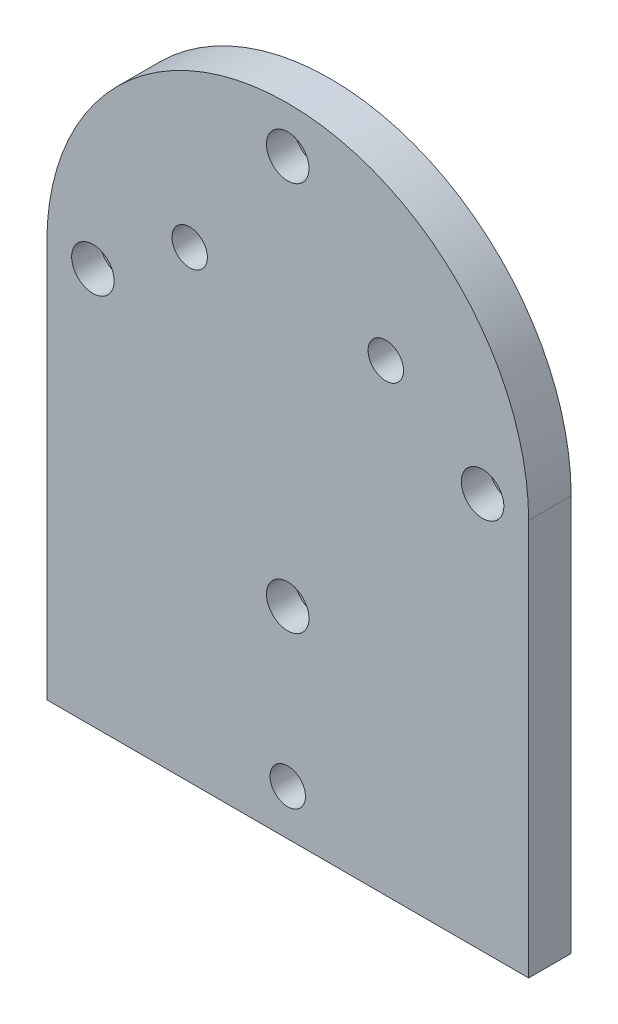
from build123d import *

# Parameters (mm, degrees)
BOSS_EXTRUDE1_DEPTH = 6
SKETCH3_R           = 3
CUT_EXTRUDE1_DEPTH  = 4
SKETCH9_R           = 2.5
CUT_EXTRUDE2_DEPTH  = 6


with BuildPart() as part:
    # Sketch2 → Boss-Extrude1 (new body)
    with BuildSketch(Plane.XY):
        with BuildLine():
            Line((2.181579686, 9.743947498), (2.181579686, -46.182702418))
            Line((2.181579686, -46.182702418), (-65.818420314, -46.182702418))
            Line((-65.818420314, -46.182702418), (-65.818420314, 9.743947498))
            ThreePointArc((-65.818420314, 9.743947498), (-31.818420314, 43.743947498), (2.181579686, 9.743947498))
        make_face()
    extrude(amount=BOSS_EXTRUDE1_DEPTH)

    # Sketch3 → Cut-Extrude1 (cut)
    with BuildSketch(Plane.XY.offset(6)):
        with Locations((-4.318420314, 9.743947498)):
            Circle(SKETCH3_R)
        with Locations((-31.818420314, -17.756052502)):
            Circle(SKETCH3_R)
        with Locations((-59.318420314, 9.743947498)):
            Circle(SKETCH3_R)
        with Locations((-31.818420314, 37.243947498)):
            Circle(SKETCH3_R)
    extrude(amount=-CUT_EXTRUDE1_DEPTH, mode=Mode.SUBTRACT)

    # Sketch9 → Cut-Extrude2 (cut)
    with BuildSketch(Plane(origin=(0, 0, 0), x_dir=(-1, 0, 0), z_dir=(0, 0, -1))):
        with Locations((45.658538984, 19.210200864)):
            Circle(SKETCH9_R)
        with Locations((17.978301644, 19.210200864)):
            Circle(SKETCH9_R)
        with Locations((31.818420314, -39.753837028)):
            Circle(SKETCH9_R)
    extrude(amount=-CUT_EXTRUDE2_DEPTH, mode=Mode.SUBTRACT)


solid = part.part
